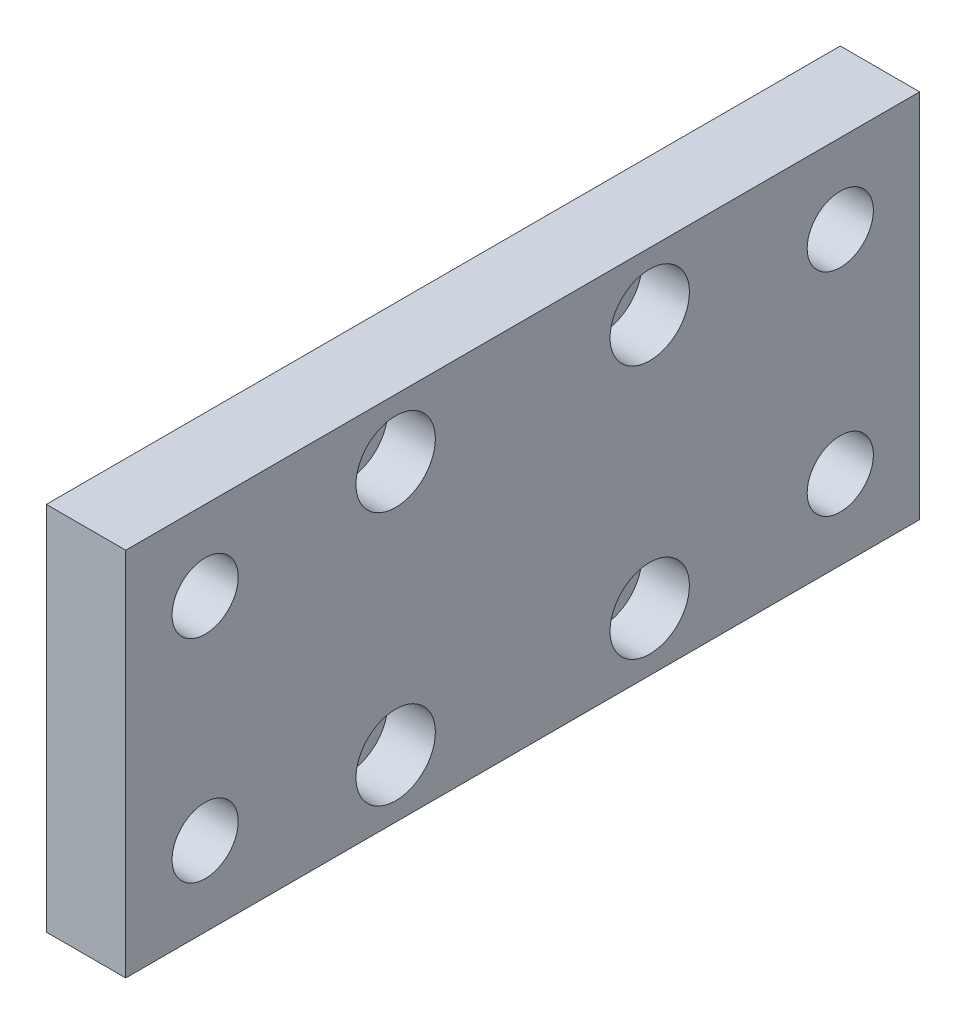
from build123d import *

# Parameters (mm, degrees)
SKETCH_1_W                = 150
SKETCH_1_H                = 70
EXTRUDE_1_DEPTH           = 15
HOLE_WIZARD_1_D           = 9
HOLE_WIZARD_1_CBORE_D     = 15
HOLE_WIZARD_1_CBORE_DEPTH = 9
HOLE_WIZARD_12_5_12_5_1_D = 12.5


with BuildPart() as part:
    # 草图1 → 凸台-拉伸1 (new body)
    with BuildSketch(Plane(origin=(0, 0, 0), x_dir=(0, 0, -1), z_dir=(1, 0, 0))):
        Rectangle(SKETCH_1_W, SKETCH_1_H)
    extrude(amount=EXTRUDE_1_DEPTH)

    # 打孔尺寸(%根据)内六角圆柱头螺钉的类型1 (through all)
    with Locations(Plane(origin=(15, 0, 0), x_dir=(0, 0, -1), z_dir=(1, 0, 0))):
        with Locations((-24, 24), (24, 24), (-24, -24), (24, -24)):
            CounterBoreHole(HOLE_WIZARD_1_D / 2, HOLE_WIZARD_1_CBORE_D / 2, HOLE_WIZARD_1_CBORE_DEPTH)

    # Ø12.5 (12.5) 直径孔1 (through all)
    with Locations(Plane.ZY):
        with Locations((-60, 20), (-60, -20), (60, 20), (60, -20)):
            Hole(HOLE_WIZARD_12_5_12_5_1_D / 2)


solid = part.part
